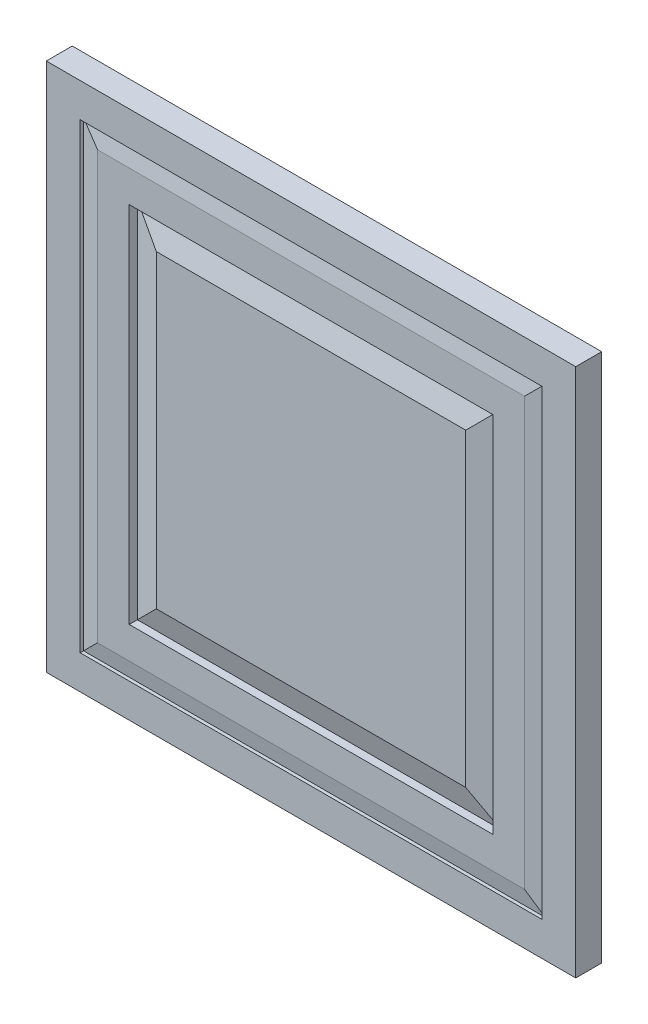
from build123d import *

# Parameters (mm, degrees)
SKETCH_1_W          = 204
SKETCH_1_H          = 204
EXTRUDE_1_DEPTH     = 10
SKETCH_6_R          = 2.5
CUT_EXTRUDE_1_DEPTH = 3
SKETCH_7_W          = 173
SKETCH_7_H          = 173
EXTRUDE_2_DEPTH     = 10


with BuildPart() as part:
    # 草图1 → 凸台-拉伸1 (new body)
    with BuildSketch(Plane.XY):
        Rectangle(SKETCH_1_W, SKETCH_1_H)
    extrude(amount=EXTRUDE_1_DEPTH)

    # 切除-扫描2: sweep along a path in 草图2
    with BuildLine(Plane.XY.offset(10)) as sweep_2_path:
        Line((-80, -80), (80, -80))
        Line((80, -80), (80, 80))
        Line((80, 80), (-80, 80))
        Line((-80, 80), (-80, -80))
    # 草图3 → 切除-扫描2 (sweep, cut)
    with BuildSketch(Plane(origin=(0, 0, 0), x_dir=(1, 0, 0), z_dir=(0, 1, 0))):
        Polygon((-88.948256764, -10), (-88.948256764, -8.70522639), (-82.270562222, -10), align=None)
    sweep(path=sweep_2_path.line, transition=Transition.RIGHT, mode=Mode.SUBTRACT)

    # 切除-扫描3: sweep along a path in 草图4
    with BuildLine(Plane.XY.offset(10)) as sweep_3_path:
        Line((-70, -70), (70, -70))
        Line((70, -70), (70, 70))
        Line((70, 70), (-70, 70))
        Line((-70, 70), (-70, -70))
    # 草图5 → 切除-扫描3 (sweep, cut)
    with BuildSketch(Plane(origin=(0, 0, 0), x_dir=(1, 0, 0), z_dir=(0, 1, 0))):
        Polygon((-70.048782141, -10), (-70.048782141, -6.864221928), (-59.608863027, -10), align=None)
    sweep(path=sweep_3_path.line, transition=Transition.RIGHT, mode=Mode.SUBTRACT)

    # 草图6 → 切除-拉伸1 (cut)
    with BuildSketch(Plane(origin=(0, 0, 0), x_dir=(-1, 0, 0), z_dir=(0, 0, -1))):
        with Locations((-92, 92)):
            Circle(SKETCH_6_R)
        with Locations((92, 92)):
            Circle(SKETCH_6_R)
        with Locations((-92, -92)):
            Circle(SKETCH_6_R)
        with Locations((92, -92)):
            Circle(SKETCH_6_R)
    extrude(amount=-CUT_EXTRUDE_1_DEPTH, mode=Mode.SUBTRACT)

    # 草图7 → 凸台-拉伸2 (add)
    with BuildSketch(Plane(origin=(0, 0, 0), x_dir=(-1, 0, 0), z_dir=(0, 0, -1))):
        Rectangle(SKETCH_7_W, SKETCH_7_H)
    extrude(amount=EXTRUDE_2_DEPTH)


solid = part.part
